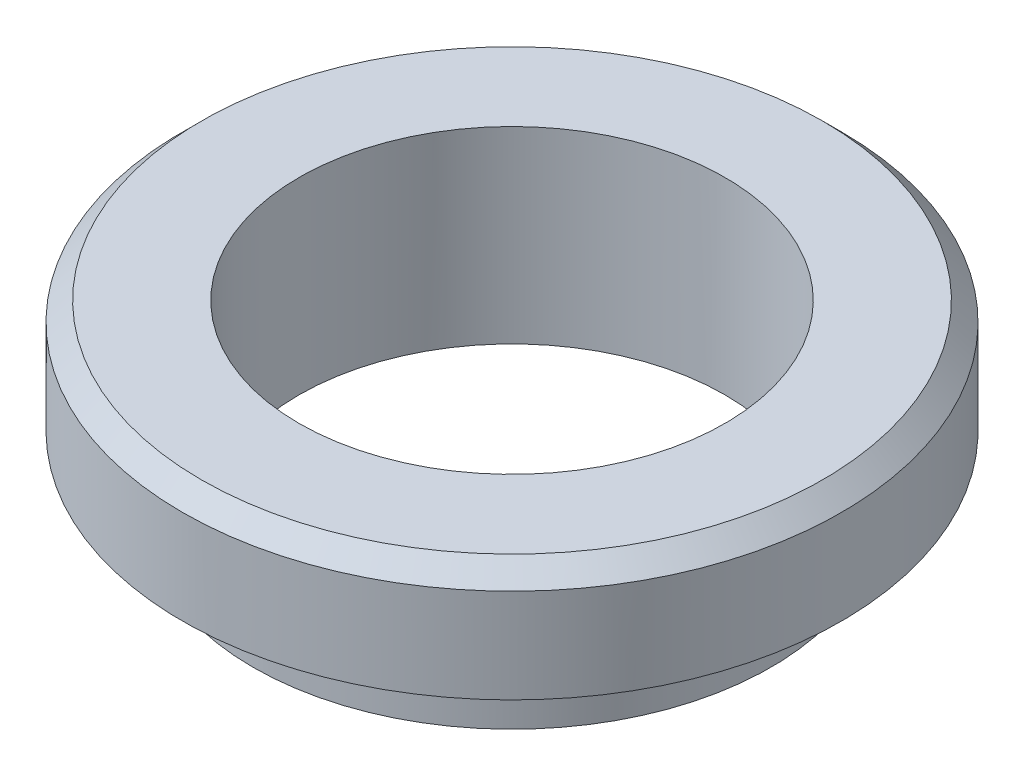
SolidWorks part; units mm, degrees
material "Q235"
ref_plane "Front Plane" through (0, 0, 0) normal (0, 0, 1) x (1, 0, 0)
ref_plane "Top Plane" through (0, 0, 0) normal (0, 1, 0) x (1, 0, 0)
ref_plane "Right Plane" through (0, 0, 0) normal (1, 0, 0) x (0, 0, -1)
sketch "Sketch1" plane through (0, 0, 0) normal (0, 0, 1) x (1, 0, 0)
  line L0 (0, 0) -> (35, 0)
  line L1 (35, 0) -> (35, -12)
  line L2 (35, -12) -> (27.5, -12)
  line L3 (27.5, -12) -> (27.5, -20)
  line L4 (27.5, -20) -> (0, -20)
  line L5 (0, -20) -> (0, 0)
  dimension "D1" = 27.5
  dimension "D2" = 35
  dimension "D3" = 8
  dimension "D4" = 12
revolve "Revolve1" add sketch "Sketch1" angle 360 about L5
hole_wizard "G1-1/2 Tapped Hole1" positions "Sketch2" profile "Sketch3" tap size "G1-1/2" standard "GB"
sketch "Sketch2" plane through (0, 0, 0) normal (0, 1, 0) x (1, 0, 0)
  point P0 (0, 0)
sketch "Sketch3" plane through (0, 0, 0) normal (1, 0, 0) x (0, 0, 1)
  line L0 (0, 0) -> (0, 116.1345)
  line L1 (0, 116.1345) -> (22.625, 102.54)
  line L2 (22.625, 102.54) -> (22.625, 0)
  line L5 (22.625, 0) -> (0, 0)
  line L10 (0, 116.1345) -> (-22.625, 102.54) construction
  line L11 (0, -6.35) -> (0, 107.95) construction
  dimension "螺纹孔钻头直径" = 45.25
  dimension "螺纹孔钻头深度" = 102.54
  dimension "导头角度" = 118
cosmetic thread "Hole cosmetic thread1"
chamfer "Chamfer1" distance 2 angle 45 1 edges at (0, 0, -35)
